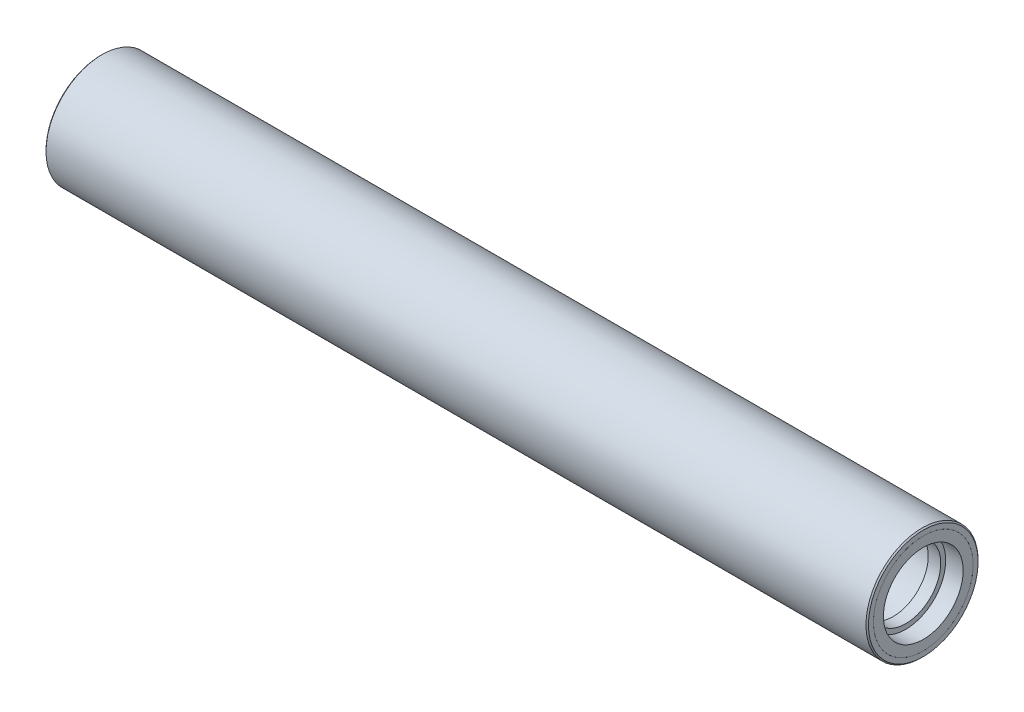
SolidWorks part; units mm, degrees
material "6061-T6 (SS)"
ref_plane "Front Plane" through (0, 0, 0) normal (0, 0, 1) x (1, 0, 0)
ref_plane "Top Plane" through (0, 0, 0) normal (0, 1, 0) x (1, 0, 0)
ref_plane "Right Plane" through (0, 0, 0) normal (1, 0, 0) x (0, 0, -1)
sketch "Sketch1" plane through (0, 0, 0) normal (0, 0, 1) x (1, 0, 0)
  line L0 (0, 0) -> (143.1309, 0) construction
  line L2 (35.1211, 17.5) -> (341.1211, 17.5)
  line L3 (23.1211, 20) -> (23.1211, 22.5)
  line L4 (23.1211, 22.5) -> (353.1211, 22.5)
  line L5 (353.1211, 20) -> (353.1211, 22.5)
  line L8 (23.1211, 20) -> (35.1211, 20)
  line L9 (35.1211, 17.5) -> (35.1211, 20)
  line L12 (353.1211, 20) -> (341.1211, 20)
  line L13 (341.1211, 17.5) -> (341.1211, 20)
  dimension "D1" = 45
  dimension "D2" = 35
  dimension "D3" = 330
  dimension "D4" = 12
  dimension "D5" = 40
revolve "Revolve1" add sketch "Sketch1" angle 360 about L0
chamfer "Chamfer1" distance 0.5 angle 45 2 edges at (353.1211, 0, 22.5) (23.1211, 0, 22.5)
sketch "Sketch2" plane through (341.1211, 0, 0) normal (1, 0, 0) x (0, 0, -1)
  circle A0 centre (0, 0) radius 20
  circle A1 centre (0, 0) radius 14
  dimension "D1" = 40
  dimension "D2" = 28
extrude "Boss-Extrude1" add sketch "Sketch2" along normal blind 12 separate body
sketch "Sketch4" plane through (353.1211, 0, 0) normal (1, 0, 0) x (0, 0, -1)
  circle A0 centre (0, 0) radius 16
  dimension "D1" = 32
extrude "Cut-Extrude1" cut sketch "Sketch4" against normal blind 7
sketch "Sketch5" plane through (35.1211, 0, 0) normal (-1, 0, 0) x (0, 0, 1)
  circle A0 centre (0, 0) radius 20
  circle A1 centre (0, 0) radius 14
  dimension "D1" = 40
  dimension "D2" = 28
extrude "Boss-Extrude2" add sketch "Sketch5" along normal blind 12 separate body
sketch "Sketch7" plane through (23.1211, 0, 0) normal (-1, 0, 0) x (0, 0, 1)
  circle A0 centre (0, 0) radius 16
  dimension "D1" = 32
extrude "Cut-Extrude2" cut sketch "Sketch7" against normal blind 7
